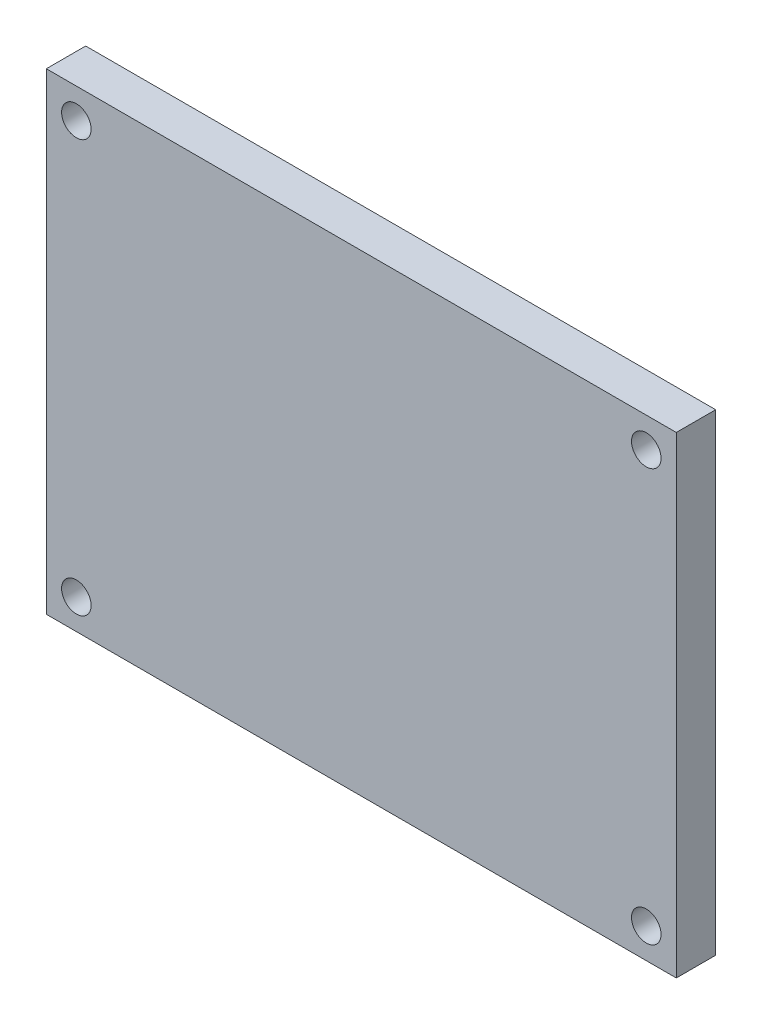
from build123d import *

# Parameters (mm, degrees)
SKETCH1_W               = 64
SKETCH1_H               = 48
BOSS_EXTRUDE1_DEPTH     = 4
CUT_EXTRUDE1_DEPTH      = 41.199502484
CUT_EXTRUDE1_DEPTH_BACK = 41.199502484
SKETCH2_R               = 1.5


with BuildPart() as part:
    # Sketch1 → Boss-Extrude1 (new body)
    with BuildSketch(Plane.XY):
        Rectangle(SKETCH1_W, SKETCH1_H)
    extrude(amount=BOSS_EXTRUDE1_DEPTH)

    # Sketch2 → Cut-Extrude1 (cut, two sides: drawn at the far end of the back side and taken through both)
    with BuildSketch(Plane.XY.offset(4).offset(-CUT_EXTRUDE1_DEPTH_BACK)):
        with Locations((28.95, -20.95)):
            Circle(SKETCH2_R)
        with Locations(Location((-28.95, -20.95, 0), (0, 0, 180))):
            Circle(SKETCH2_R)
        with Locations(Location((28.95, 20.95, 0), (0, 0, 180))):
            Circle(SKETCH2_R)
        with Locations((-28.95, 20.95)):
            Circle(SKETCH2_R)
    extrude(amount=CUT_EXTRUDE1_DEPTH + CUT_EXTRUDE1_DEPTH_BACK, mode=Mode.SUBTRACT)


solid = part.part
